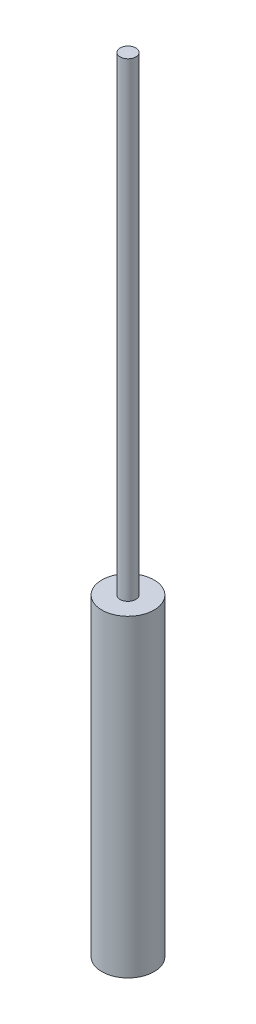
SolidWorks part; units mm, degrees
ref_plane "Front Plane" through (0, 0, 0) normal (0, 0, 1) x (1, 0, 0)
ref_plane "Top Plane" through (0, 0, 0) normal (0, 1, 0) x (1, 0, 0)
ref_plane "Right Plane" through (0, 0, 0) normal (1, 0, 0) x (0, 0, -1)
sketch "Sketch1" plane through (0, 0, 0) normal (0, 1, 0) x (1, 0, 0)
  circle A0 centre (0, 0) radius 5
  dimension "D1" = 10
extrude "Boss-Extrude1" add sketch "Sketch1" along normal blind 60
sketch "Sketch2" plane through (0, 60, 0) normal (0, 1, 0) x (1, 0, 0)
  circle A0 centre (0, 0) radius 1.5
  dimension "D1" = 3
extrude "Boss-Extrude2" add sketch "Sketch2" along normal blind 90
hole_wizard "M4 Tapped Hole1" positions "Sketch3" profile "Sketch4" tap size "M4" standard "GB"
sketch "Sketch3" plane through (0, 0, 0) normal (0, -1, 0) x (-1, 0, 0)
  point P0 (0, 0)
sketch "Sketch4" plane through (0, 0, 0) normal (1, 0, 0) x (0, 0, -1)
  line L0 (0, 0) -> (0, 12.4914)
  line L1 (0, 12.4914) -> (1.65, 11.5)
  line L2 (1.65, 11.5) -> (1.65, 0.375)
  line L3 (1.65, 0.375) -> (2.025, 0)
  line L5 (2.025, 0) -> (0, 0)
  line L6 (-1.65, 0.375) -> (-2.025, 0) construction
  line L10 (0, 12.4914) -> (-1.65, 11.5) construction
  line L11 (0, -6.35) -> (0, 107.95) construction
  dimension "螺纹孔钻头直径" = 3.3
  dimension "螺纹孔钻头深度" = 11.5
  dimension "近端锥形沉头孔直径" = 4.05
  dimension "近端锥形沉头孔角度" = 90
  dimension "导头角度" = 118
cosmetic thread "Cosmetic Thread1" parameters "D1"=8, "D2"=4
